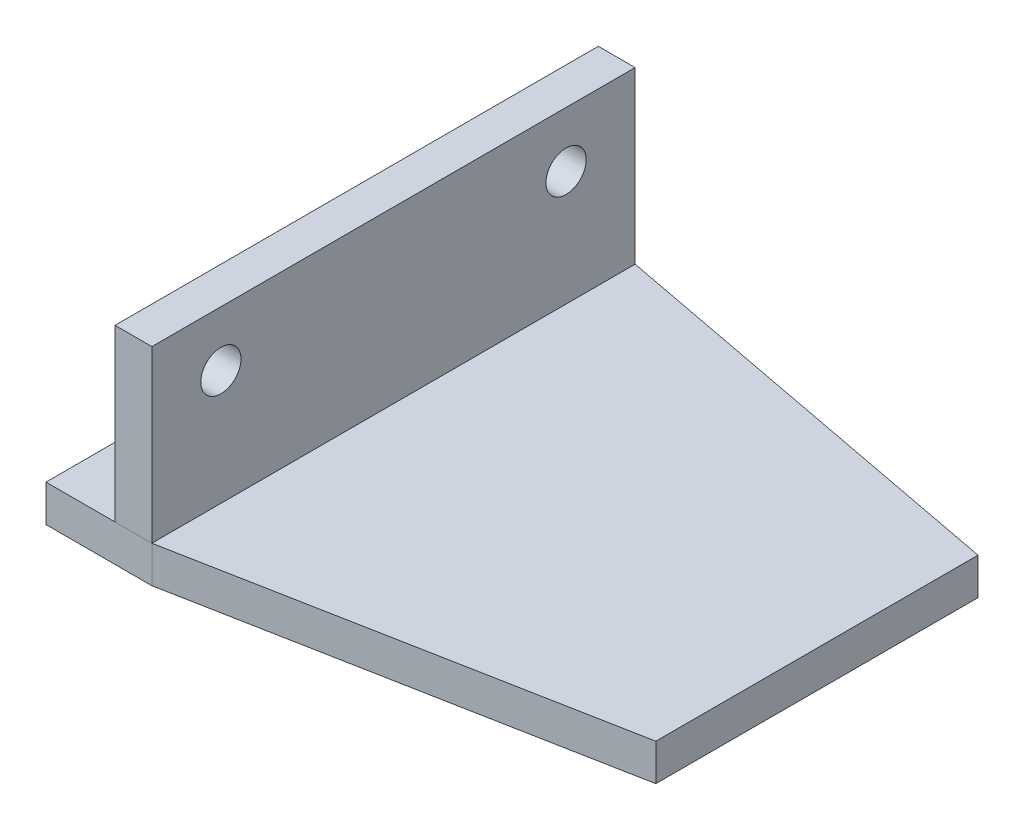
SolidWorks part; units mm, degrees
material "A3"
ref_plane "前视基准面" through (0, 0, 0) normal (0, 0, 1) x (1, 0, 0)
ref_plane "上视基准面" through (0, 0, 0) normal (0, 1, 0) x (1, 0, 0)
ref_plane "右视基准面" through (0, 0, 0) normal (1, 0, 0) x (0, 0, -1)
sketch "草图1" plane through (0, 0, 0) normal (0, 1, 0) x (1, 0, 0)
  line L0 (0, 0) -> (230, 0) construction
  line L1 (230, -70) -> (230, 70)
  line L2 (230, 70) -> (46, 105)
  line L3 (46, 105) -> (0, 105)
  line L4 (0, 105) -> (0, -105)
  line L5 (46, -105) -> (0, -105)
  line L6 (230, -70) -> (46, -105)
  dimension "D1" = 210
  dimension "D2" = 140
  dimension "D3" = 230
  dimension "D4" = 46
extrude "凸台-拉伸1" add sketch "草图1" along normal blind 16
sketch "草图2" plane through (0, 16, 0) normal (0, 1, 0) x (1, 0, 0)
  line L0 (0, -105) -> (46, -105) construction
  line L1 (46, 105) -> (30, 105)
  line L2 (46, 105) -> (46, -105)
  line L3 (46, -105) -> (30, -105)
  line L4 (30, 105) -> (30, -105)
  dimension "D1" = 16
extrude "凸台-拉伸2" add sketch "草图2" along normal blind 74 separate body
hole_wizard "M20 螺纹孔1" positions "草图3" profile "草图4" tap size "M20" standard "GB"
sketch "草图3" plane through (30, 0, 0) normal (-1, 0, 0) x (0, 0, 1)
  line L0 (0, 0) -> (0, 90) construction
  line L1 (-105, 90) -> (105, 90) construction
  line L3 (-105, 16) -> (105, 16) construction
  point P1 (-75, 66)
  point P13 (75, 66)
  dimension "D1" = 150
  dimension "D2" = 50
sketch "草图4" plane through (30, 66, -75) normal (0, 1, 0) x (0, 0, 1)
  line L0 (0, 0) -> (0, 57.7575)
  line L1 (0, 57.7575) -> (8.75, 52.5)
  line L2 (8.75, 52.5) -> (8.75, 0)
  line L5 (8.75, 0) -> (0, 0)
  line L10 (0, 57.7575) -> (-8.75, 52.5) construction
  line L11 (0, -6.35) -> (0, 107.95) construction
  dimension "螺纹孔钻头直径" = 17.5
  dimension "螺纹孔钻头深度" = 52.5
  dimension "导头角度" = 118
cosmetic thread "孔螺蚊线1"
cosmetic thread "孔螺蚊线2"
